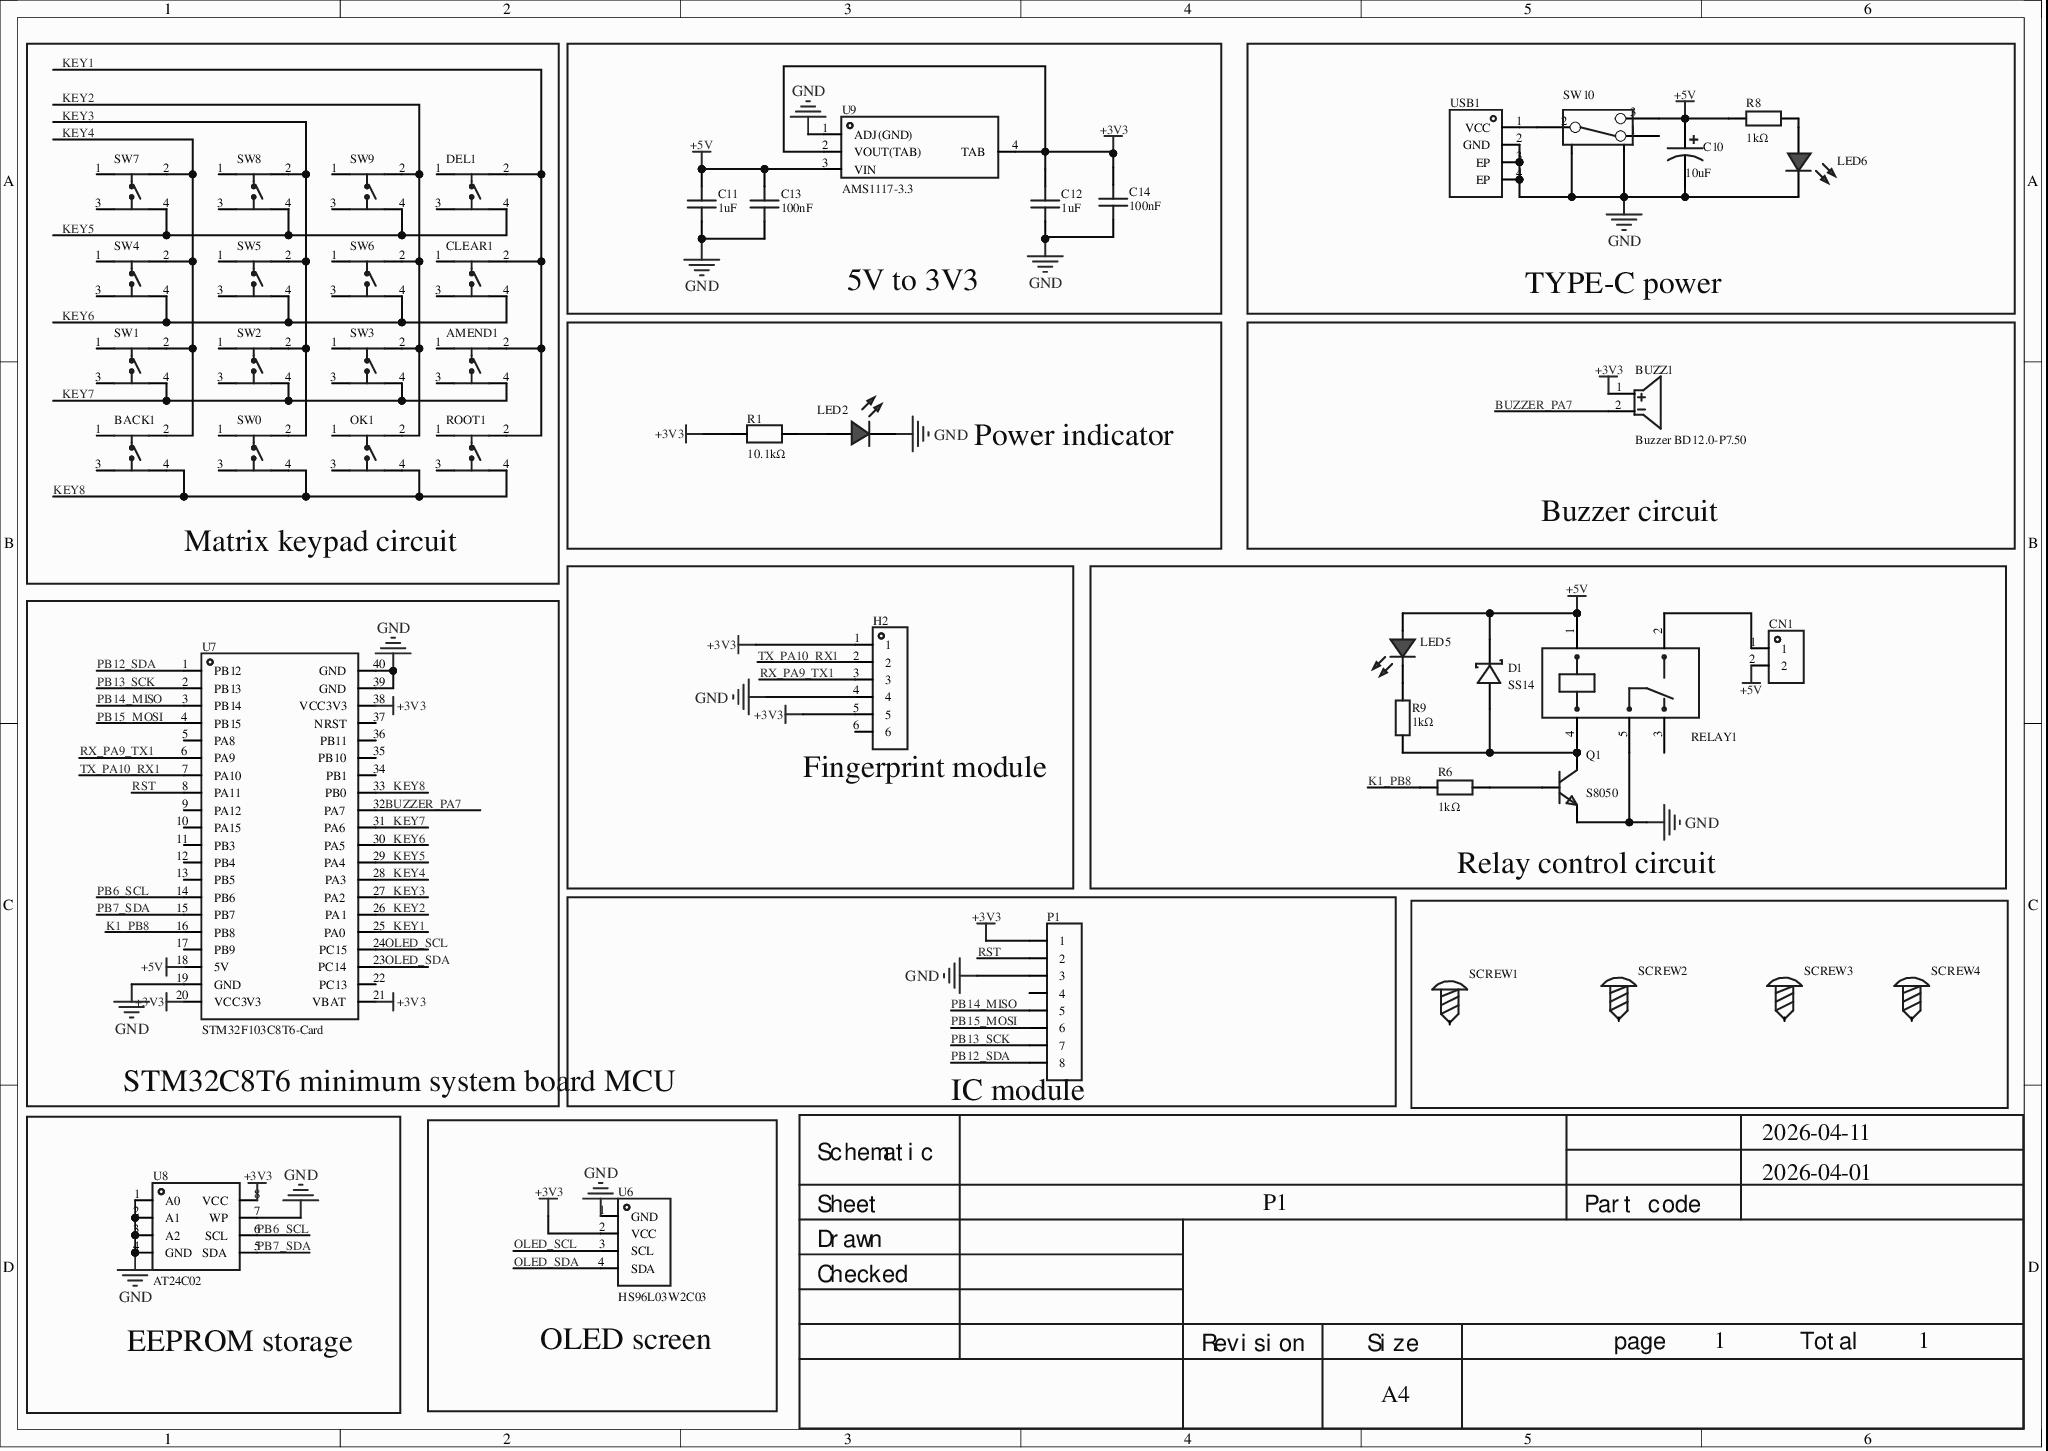
[diagram p0: MISC61668-2.schdoc]
# Altium project MISC61668-3.PrjPcb
1 sheet, 45 parts. Net scope: global (net labels, ports and power ports of the same name join across sheets).
Board file: MISC61668.pcbdoc

## Sheet MISC61668-2.schdoc
size 297 x 210 mm; Version: V1.0; @Project Name: MISC61668; @Page Count: 1; @Update Date: 2026-04-11; @Create Date: 2026-04-11; @Schematic Name: MISC61668; @Page No: 1

### Parts
AMEND1  KH-6X6X5H-STM  [SW-SMD_4P-L6.0-W6.0-P4.50-LS9.0-2]  (value not drawn)
BACK1  KH-6X6X5H-STM  [SW-SMD_4P-L6.0-W6.0-P4.50-LS9.0-2]  (value not drawn)
BUZZ1  Buzzer BD12.0-P7.50  [BUZ-TH_BD12.0-P7.50-D0.6-FD]
C10  10uF  [CAP-TH_BD5.0-P2.00-D0.8-FD]
C11  1uF  [C0603]
C12  1uF  [C0603]
C13  100nF  [C0603]
C14  100nF  [C0603]
CLEAR1  KH-6X6X5H-STM  [SW-SMD_4P-L6.0-W6.0-P4.50-LS9.0-2]  (value not drawn)
CN1  ZX-XH2.54-2PZZ  [CONN-TH_2P-P2.50_HX25003-2A]  (value not drawn)
D1  SS14  [SMA_L4.2-W2.6-LS5.3-RD]
DEL1  KH-6X6X5H-STM  [SW-SMD_4P-L6.0-W6.0-P4.50-LS9.0-2]  (value not drawn)
H2  PM254V-11-06-H85  [hdr-th_6p-p2.54-v-f]  (value not drawn)
LED2  (no value)  [LED-TH_5mm]
LED5  XL-302SURD  [LED-TH_BD3.8-P2.54-RD]  (value not drawn)
LED6  (no value)  [LED-TH_5mm]
OK1  KH-6X6X5H-STM  [SW-SMD_4P-L6.0-W6.0-P4.50-LS9.0-2]  (value not drawn)
P1  2.54-1*8P female, RoHS  [HDR-TH_8P-P2.54-V-F-1]  (value not drawn)
Q1  S8050  [SOT-23-3_L2.9-W1.6-P1.90-LS2.8-BR]
R1  10.1kΩ  [R0805]
R6  1kΩ  [R0603]
R8  1kΩ  [RES-TH_BD2.5-L6.5-P10.50-D0.6]
R9  1kΩ  [RES-TH_BD2.5-L6.5-P10.50-D0.6]
RELAY1  SRD-12VDC-SL-C  [RELAY-TH_SRD-XXVDC-XL-C]  (value not drawn)
ROOT1  KH-6X6X5H-STM  [SW-SMD_4P-L6.0-W6.0-P4.50-LS9.0-2]  (value not drawn)
SCREW1  (no value)  [M3螺丝]
SCREW2  (no value)  [M3螺丝]
SCREW3  (no value)  [M3螺丝]
SCREW4  (no value)  [M3螺丝]
SW0  KH-6X6X5H-STM  [SW-SMD_4P-L6.0-W6.0-P4.50-LS9.0-2]  (value not drawn)
SW1  KH-6X6X5H-STM  [SW-SMD_4P-L6.0-W6.0-P4.50-LS9.0-2]  (value not drawn)
SW2  KH-6X6X5H-STM  [SW-SMD_4P-L6.0-W6.0-P4.50-LS9.0-2]  (value not drawn)
SW3  KH-6X6X5H-STM  [SW-SMD_4P-L6.0-W6.0-P4.50-LS9.0-2]  (value not drawn)
SW4  KH-6X6X5H-STM  [SW-SMD_4P-L6.0-W6.0-P4.50-LS9.0-2]  (value not drawn)
SW5  KH-6X6X5H-STM  [SW-SMD_4P-L6.0-W6.0-P4.50-LS9.0-2]  (value not drawn)
SW6  KH-6X6X5H-STM  [SW-SMD_4P-L6.0-W6.0-P4.50-LS9.0-2]  (value not drawn)
SW7  KH-6X6X5H-STM  [SW-SMD_4P-L6.0-W6.0-P4.50-LS9.0-2]  (value not drawn)
SW8  KH-6X6X5H-STM  [SW-SMD_4P-L6.0-W6.0-P4.50-LS9.0-2]  (value not drawn)
SW9  KH-6X6X5H-STM  [SW-SMD_4P-L6.0-W6.0-P4.50-LS9.0-2]  (value not drawn)
SW10  SK-12E12-G5  [SW-TH_SK-12E12-G5]  (value not drawn)
U6  HS96L03W2C03  [OLED-TH_L27.8-W27.2-P2.54_C9900033791]
U7  STM32F103C8T6-Card  [CONN-TH_L53.3-W22.9_STM32F103C8T6-CARD]
U8  AT24C02  [SOP-8_L5.0-W4.0-P1.27-LS6.0-BL]
U9  AMS1117-3.3  [SOT-223-4_L6.5-W3.5-P2.30-LS7.0-BR]
USB1  KH-TYPE-C-2P  [USB-SMD_KH-TYPE-C-2P]  (value not drawn)

### Blocks framed on the sheet
Matrix keypad circuit: AMEND1 BACK1 CLEAR1 DEL1 OK1 ROOT1 SW0-SW9
5V to 3V3: C11-C14 U9
TYPE-C power: C10 LED6 R8 SW10 USB1
Power indicator: LED2 R1
Fingerprint module: H2
STM32C8T6 minimum system board MCU: U7
IC module: P1
Relay control circuit: SCREW1-SCREW4
OLED screen: U6

### Nets
+3V3: BUZZ1.1 C12.2 C14.2 H2.1 H2.5 P1.1 R1.1 U6.2(VCC) U7.20(VCC3V3) U7.21(VBAT) U7.38(VCC3V3) U8.8(VCC) U9.2(VOUT(TAB)) U9.4(TAB)
+5V: C10.1 C11.2 C13.2 CN1.2 D1.1(K) LED5.2(A) R8.1 RELAY1.1 SW10.3 U7.18(5V) U9.3(VIN)
GND: C10.2 C11.1 C12.1 C13.1 C14.1 H2.4 LED2.2(A) LED6.2(A) P1.3 Q1.2 RELAY1.5 SW10.4 SW10.5 U6.1(GND) U7.19(GND) U7.39(GND) U7.40(GND) U8.1(A0) U8.2(A1) U8.3(A2) U8.4(GND) U8.7(WP) U9.1(ADJ(GND)) USB1.2(GND) USB1.3(EP) USB1.4(EP)
BUZZER_PA7: BUZZ1.2 U7.32(PA7)
K1_PB8: R6.2 U7.16(PB8)
KEY1: AMEND1.2 CLEAR1.2 DEL1.2 ROOT1.2 U7.25(PA0)
KEY2: OK1.2 SW3.2 SW6.2 SW9.2 U7.26(PA1)
KEY3: SW0.2 SW2.2 SW5.2 SW8.2 U7.27(PA2)
KEY4: BACK1.2 SW1.2 SW4.2 SW7.2 U7.28(PA3)
KEY5: DEL1.4 SW7.4 SW8.4 SW9.4 U7.29(PA4)
KEY6: CLEAR1.4 SW4.4 SW5.4 SW6.4 U7.30(PA5)
KEY7: AMEND1.4 SW1.4 SW2.4 SW3.4 U7.31(PA6)
KEY8: BACK1.4 OK1.4 ROOT1.4 SW0.4 U7.33(PB0)
OLED_SCL: U6.3(SCL) U7.24(PC15)
OLED_SDA: U6.4(SDA) U7.23(PC14)
PB6_SCL: U7.14(PB6) U8.6(SCL)
PB7_SDA: U7.15(PB7) U8.5(SDA)
PB12_SDA: P1.8 U7.1(PB12)
PB13_SCK: P1.7 U7.2(PB13)
PB14_MISO: P1.5 U7.3(PB14)
PB15_MOSI: P1.6 U7.4(PB15)
RST: P1.2 U7.8(PA11)
RX_PA9_TX1: H2.3 U7.6(PA9)
TX_PA10_RX1: H2.2 U7.7(PA10)
NetCN1_1: CN1.1 RELAY1.2
NetD1_2: D1.2(A) Q1.3 R9.1 RELAY1.4
NetLED2_1: LED2.1(C) R1.2
NetLED5_1: LED5.1(K) R9.2
NetLED6_1: LED6.1(C) R8.2
NetQ1_1: Q1.1 R6.1
NetSW10_2: SW10.2 USB1.1(VCC)

Not connected (* = marked no-connect by the designer): AMEND1 1* 3*; BACK1 1* 3*; CLEAR1 1* 3*; DEL1 1* 3*; H2 6*; OK1 1* 3*; P1 4*; RELAY1 3*; ROOT1 1* 3*; SCREW1 1*; SCREW2 1*; SCREW3 1*; SCREW4 1*; SW0 1* 3*; SW1 1* 3*; SW2 1* 3*; SW3 1* 3*; SW4 1* 3*; SW5 1* 3*; SW6 1* 3*; SW7 1* 3*; SW8 1* 3*; SW9 1* 3*; SW10 1*; U7 5(PA8)* 9(PA12)* 10(PA15)* 11(PB3)* 12(PB4)* 13(PB5)* 17(PB9)* 22(PC13)* 34(PB1)* 35(PB10)* 36(PB11)* 37(NRST)*

### Notes on the sheet
- Buzzer circuit
- EEPROM storage
- 2026-04-11
- Schematic
- Sheet
- P1
- Part code
- 2026-04-01
- Checked
- Drawn
- Revision
- Size
- A4
- page
- 1
- Total

### Library data of the parts
AMEND1 BACK1 CLEAR1 DEL1 OK1 ROOT1 SW0-SW9 = KH-6X6X5H-STM: 电路结构:单刀单掷;按钮形状:圆形按钮;安装方式:立贴;开关长度:6mm;开关宽度:6mm;开关高度:5mm;带支架:不带;触点电流:50mA;额定电压(DC):12V;机械寿命:8万次;; Manufacturer: kinghelm(金航标); AddInBom: yes; ModelId: fbf4ceca6c4742d48614ab6a891ef981; ModelName: SW-SMD_4P-L6.0-W6.0-P4.50-LS11.0; ModelTransform: 330.708,251.968,0,0,0,0,0,-0.005,0; Circuit: SPST; Actuator Style: Round button; Switch Length: 6mm; Switch Height: 5mm; Strike Gundam: Without; Contact Current: 50mA; Voltage Rating (DC): 12V; Actuator/Cap Color: Black; Pin Style: Gull-wing; Mechanical Life: 8 ten-thousand cycles; Symbol: KH-6X6X5H-STM; Device: KH-6X6X5H-STM; LCSC Part Name: 6*6*5mm 立贴 轻触开关; SupplierPart: C2837531; ManufacturerPart: KH-6X6X5H-STM; Supplier Footprint: SMD; JLCPCB Part Class: Extended library; Datasheet: https://atta.szlcsc.com/upload/public/pdf/source/20210608/C2837531_45E87AB996CE723B09405FF2EA209C4C.pdf; Supplier: LCSC; ConvertToPcb: yes; FootprintName: SW-SMD_4P-L6.0-W6.0-P4.50-LS9.0-2; Mounting Style: SMD; Switch Width: 6mm
BUZZ1 = 蜂鸣器BD12.0-P7.50: AddInBom: yes; ModelId: 0e4a13d1d30a43b48b3e728a221f21ea; ModelTransform: 472.44,472.32441,0,0,0,0,0,0,-137.795; Symbol: Buzzer BD12.0-P7.50; Device: Buzzer BD12.0-P7.50; LCSC Part Name: 蜂鸣器BD12.0-P7.50; SupplierPart: C9900003117; ManufacturerPart: 蜂鸣器BD12.0-P7.50; Supplier Footprint: TH-BD12.0-P7.50-D0.6; JLCPCB Part Class: Extended library; Supplier: LCSC; ConvertToPcb: yes; FootprintName: BUZ-TH_BD12.0-P7.50-D0.6-FD; ModelName: BUZ-TH_BD12.0-P7.50-D0.6-FD
C10 = 01EC1809SHC10UF50V: Capacitance: 10uF; tolerance: ±20%; rated voltage: 50V; ripple current: 50mA@120Hz; ESR: -;; Manufacturer: KNSCHA(科尼盛); AddInBom: yes; ModelId: edeeed87cbc746108d01291548c38636; ModelName: CAP-TH_D5.0×H7.0×P2.0; ModelTransform: 197.091,196.7911,0,0,0,0,0,0,-137.795; φD: 5mm; L: 11mm; Lifetime @ Temp: 5000hrs@105℃; Symbol: 01EC1809SHC10UF50V; Device: 01EC1809SHC10UF50V; LCSC Part Name: 10uF ±20% 50V; SupplierPart: C503219; ManufacturerPart: 01EC1809SHC10UF50V; Supplier Footprint: 插件,D5xL11mm; JLCPCB Part Class: Extended library; Datasheet: https://atta.szlcsc.com/upload/public/pdf/source/20200324/C503219_39D1683F20D4DB1C41D8BE9142629697.pdf; Supplier: LCSC; ConvertToPcb: yes; FootprintName: CAP-TH_BD5.0-P2.00-D0.8-FD; Value: 10uF; Tolerance: ±20%; Rated Voltage: 50V; Ripple Current: 50mA@120Hz; Equivalent Series Resistance(ESR): -; Lead Spacing: 2mm
C11 C12 = CL10A105KB8NNNC: Capacitance: 1uF; tolerance: ±10%; rated voltage: 50V; dielectric (temperature coefficient): X5R;; Manufacturer: SAMSUNG(三星); AddInBom: yes; ModelId: ac125912035d415993ca9572d50418b1; ModelName: C0603_L1.6-W0.8-H0.8; ModelTransform: 62.992,31.496,0,0,0,0,0,0,0; Symbol: CL10A105KB8NNNC; Device: CL10A105KB8NNNC; LCSC Part Name: 1uF ±10% 50V; SupplierPart: C15849; ManufacturerPart: CL10A105KB8NNNC; Supplier Footprint: 0603; JLCPCB Part Class: Basic library; Datasheet: https://atta.szlcsc.com/upload/public/pdf/source/20160218/1457707763339.pdf; Supplier: LCSC; ConvertToPcb: yes; FootprintName: C0603; Value: 1uF; Tolerance: ±10%; Voltage Rated: 50V; Temperature Coefficient: X5R
C13 C14 = CC0603KRX7R9BB104: Capacitance: 100nF; tolerance: ±10%; rated voltage: 50V; dielectric (temperature coefficient): X7R;; Manufacturer: YAGEO(国巨); AddInBom: yes; ModelId: ac125912035d415993ca9572d50418b1; ModelName: C0603_L1.6-W0.8-H0.8; ModelTransform: 62.992,31.496,0,0,0,0,0,0,0; Symbol: CC0603KRX7R9BB104; Device: CC0603KRX7R9BB104; Supplier: LCSC; Manufacturer Part: CC0603KRX7R9BB104; Value: 100nF; Supplier Part: C14663; JLCPCB Part Class: Basic library; LCSC Part Name: 100nF ±10% 50V; Supplier Footprint: 0603; Datasheet: https://atta.szlcsc.com/upload/public/pdf/source/20180910/C282072_33301C7F631E79921B82A8DAC6BCC5B3.pdf; ConvertToPcb: yes; FootprintName: C0603; Tolerance: ±10%; Voltage Rated: 50V; Temperature Coefficient: X7R
CN1 = ZX-XH2.54-2PZZ: 插针结构:1x2P;间距:2.54mm;安装方式:直插;参考系列:XH;总PIN数:2P;排数:1;每排PIN数:2;行距:-;额定电流:3A;触头材质:黄铜;触头镀层:锡;工作温度范围:-25℃~+85℃;; Manufacturer: Megastar(兆星); AddInBom: yes; ModelId: 17c7be61cc0b4bc5acccb67e71c47088; ModelTransform: 295.275,232.283,0,180,0,0,0,-21.654,-129.921; Pins Structure: 1x2P; Pitch: 2.54mm; Reference Series: XH; Number of PINs Per Row: 2; Current Rating (Max): 3A; Symbol: ZX-XH2.54-2PZZ; Device: ZX-XH2.54-2PZZ; LCSC Part Name: ZX-XH2.54-2PZZ; SupplierPart: C7429632; ManufacturerPart: ZX-XH2.54-2PZZ; Supplier Footprint: 插件,P=2.54mm; JLCPCB Part Class: Extended library; Datasheet: https://atta.szlcsc.com/upload/public/pdf/source/20230619/19BA6947230AA44A04D3EDD65E618FD0.pdf; Supplier: LCSC; ConvertToPcb: yes; FootprintName: CONN-TH_2P-P2.50_HX25003-2A; ModelName: CONN-TH_2P-P2.50_HX25003-2A; Mounting Style: Through-hole; Number of Pins: 2P; Number of Rows: 1; Row Spacing: -; Contact Material: Brass; Contact Plating: Tin; Operating Temperature Range: -25℃~+85℃
D1 = SS14_C2480: Diode configuration: independent; forward voltage (Vf): 550mV@1A; DC reverse voltage (Vr): 40V; rectifier current: 1A;; Manufacturer: MDD(辰达半导体); AddInBom: yes; ModelId: c9e8185d46a94015b9fa58a531b156cf; ModelTransform: 204.83943,103.346,0,0,0,0,-0.001,0.001,0; Reverse Leakage Current (Ir): 300uA@40V; Symbol: SS14; Device: SS14_C2480; LCSC Part Name: 电压:40V 电流:1A; SupplierPart: C2480; ManufacturerPart: SS14; Supplier Footprint: SMA(DO-214AC); JLCPCB Part Class: Basic library; Datasheet: https://atta.szlcsc.com/upload/public/pdf/source/20240710/EF24798823EE33D63F154ED67BAC5E71.pdf; Supplier: LCSC; ConvertToPcb: yes; FootprintName: SMA_L4.2-W2.6-LS5.3-RD; ModelName: SMA_L4.2-W2.6-LS5.3-RD; Diode Configuration: Independent; Forward Voltage (Vf@If): 550mV@1A; Reverse Voltage (Vr): 40V; Rectified Current: 1A
H2 = PM254V-11-06-H85: 插孔结构:1x6P;间距:2.54mm;行距:-;圆孔/方孔:方孔;安装类型:直插;排数:单排;总孔位数:6P;额定电流:3A;额定电压:250V;插孔方向:顶部;塑高:-;工作温度范围:-40℃~+105℃;; Manufacturer: XFCN(兴飞); Check: false; AddInBom: yes; ModelId: 0f5bcf94dcda47d085f24cdca1696fe9; ModelTransform: 619.684,94.488,0,0,0,0,0,0,-125.984; Holes Structure: 1x6P; Pitch: 2.54mm; Circular Hole / Square Hole: Square hole; Number of Holes: 6P; Current Rating (Max): 3A; Voltage Rating (Max): 250V; Holes Direction: Top; Symbol: PM254V-11-06-H85; Device: PM254V-11-06-H85; Supplier: LCSC; Supplier Part: C2832269; Manufacturer Part: PM254V-11-06-H85; JLCPCB Part Class: Extended library; LCSC Part Name: 间距:2.54mm 1x6P 直插; Supplier Footprint: 插件,P=2.54mm; Datasheet: https://atta.szlcsc.com/upload/public/pdf/source/20210514/C2832269_B3EC97736B37C2783BDCE3050AA57447.pdf; ConvertToPcb: yes; FootprintName: hdr-th_6p-p2.54-v-f; ModelName: HDR-TH_6P-P2.54-V-F; Row Spacing: -; Mounting Type: Through-hole; Number of Rows: Single row; Insulation Height: -; Operating Temperature Range: -40℃~+105℃
LED2 LED6 = LED_TH-R_5mm: ConvertToPcb: yes; ModelId: fe9cea1bdf7642cd8d9a5077ed0e2b58; ModelName: LED-TH_BD5.9-P2.54-RD_RED; ModelTransform: 222.16,238.98,581.81,180,0,0,-6,0,-220; Symbol: LED_TH-R; Device: LED_TH-R_5mm; AddInBom: yes; FootprintName: LED-TH_5mm; Supplier Footprint: 插件
LED5 = XL-302SURD: 灯头类型:3mm圆形灯头;发光颜色:红色;功率:80mW;正向电流:30mA;主波长:615nm~620nm;透镜颜色:红色透镜;色温:-;发光角度:50°;载带方式:-;工作温度:-25℃~+85℃;; Manufacturer: XINGLIGHT(成兴光); AddInBom: yes; Lamp Holder Type: 3mm round lamp holder; Emitted Color: Red; Power Dissipation: 80mW; Forward Current: 30mA; Peak Wavelength: 625nm; Lens Color: Red lens; Viewing Angle: 50°; ModelId: 6a9b7f7cc45d49ea908a5f911cd0be96; ModelTransform: 134.372,149.6,0,180,0,0,6.89,0,-196.85; Symbol: XL-302SURD; Device: XL-302SURD; LCSC Part Name: XL-302SURD; SupplierPart: C2895470; ManufacturerPart: XL-302SURD; Supplier Footprint: 插件,D=3mm; JLCPCB Part Class: Extended library; Datasheet: https://atta.szlcsc.com/upload/public/pdf/source/20240112/E1E2B82945FD635E4907401DDE6D4922.pdf; Supplier: LCSC; ConvertToPcb: yes; Dominant Wavelength: 615nm~620nm; Color Temperature: -; Mounting Sytle: -; Operating Temperature: -25℃~+85℃; FootprintName: LED-TH_BD3.8-P2.54-RD; ModelName: LED-TH_BD3.8-P2.54-RD
P1 = 2.54-1*8P母环保: Socket structure: 1x8P; pitch: 2.54mm; row spacing: -; mounting type: through-hole; rows: single row; total positions: 8P; plastic height: -; contact material: -; contact plating: -;; Manufacturer: BOOMELE(博穆精密); Symbol: Header-Female-2.54_1x8; AddInBom: yes; ModelId: 0f7e4d9227ef4fa08d5469c22cc70cdb; ModelName: HDR-F-2.54_1x8; ModelTransform: 799.99844,100,0,0,0,0,0,0,-118.11; Device: 2.54-1*8P female, RoHS; LCSC Part Name: 间距:2.54mm 1x8P 直插; SupplierPart: C27438; ManufacturerPart: 2.54-1*8P母环保; Supplier Footprint: 插件,P=2.54mm; JLCPCB Part Class: Extended library; Datasheet: https://atta.szlcsc.com/upload/public/pdf/source/20231221/1CA800C6799ED97958773716FAA1BFFE.pdf; Supplier: LCSC; ConvertToPcb: yes; FootprintName: HDR-TH_8P-P2.54-V-F-1; Holes Structure: 1x8P; Pitch: 2.54mm; Row Spacing: -; Mounting Type: Through-hole; Number of Rows: Single row; Number of Holes: 8P; Insulation Height: -; Contact Material: -; Contact Plating: -
Q1 = S8050_C181158: Transistor type: NPN; collector current (Ic): 500mA; collector-emitter breakdown voltage (Vceo): 25V; power (Pd): 300mW;; Manufacturer: Hottech(合科泰); AddInBom: yes; ModelId: 89cb27a44ab2466697082bb9fd73a7d0; ModelName: SOT-23-3L_L2.9-W1.6-H1.1-LS2.8-P0.95; ModelTransform: 114.173,110.236,0,90,0,0,0,0,0; Transition Frequency (fT): 150MHz; Collector Cut-Off Current (Icbo): 100nA; Collector-Emitter Saturation Voltage (VCE(sat)@Ic,Ib): 600mV@500mA,50mA; Symbol: S8050_C181158; Device: S8050_C181158; LCSC Part Name: NPN 电流:500mA 耐压:25V; SupplierPart: C181158; ManufacturerPart: S8050; Supplier Footprint: SOT-23; JLCPCB Part Class: Extended library; Datasheet: https://atta.szlcsc.com/upload/public/pdf/source/20220506/D987F39D56F2975D34EC7947E75C4ABC.pdf; Supplier: LCSC; ConvertToPcb: yes; FootprintName: SOT-23-3_L2.9-W1.6-P1.90-LS2.8-BR; Transistor Type: NPN; Collector Current (Ic): 500mA; Collector-Emitter Breakdown Voltage (Vceo): 25V; Power Dissipation (Pd): 300mW; Operating Temperature: -
R1 = RT0805BRD0710K1L: Resistor type: thin film; resistance: 10.1kΩ; tolerance: ±0.1%; power: 125mW; temperature coefficient: ±25ppm/℃;; Manufacturer: YAGEO(国巨); AddInBom: yes; ModelId: 37a81e68749a4138bd2dfa6897b24b85; ModelName: R0805_L2.0-W1.3-H0.6; ModelTransform: 78.74,51.181,0,0,0,0,0,-0.0005,0; Symbol: RT0805BRD0710K1L; Device: RT0805BRD0710K1L; LCSC Part Name: 薄膜电阻 10.1kΩ ±0.1% 125mW; SupplierPart: C865133; ManufacturerPart: RT0805BRD0710K1L; Supplier Footprint: 0805; JLCPCB Part Class: Extended library; Datasheet: https://atta.szlcsc.com/upload/public/pdf/source/20200610/C326738_5639A9F1B6EB6E4AE2197577D3456E7F.pdf; Supplier: LCSC; ConvertToPcb: yes; FootprintName: R0805; Type: Thin film resistor; Value: 10.1kΩ; Tolerance: ±0.1%; Power(Watts): 125mW; Temperature Coefficient: ±25ppm/℃; Operating Temperature Range: -55℃~+155℃
R6 = RC0603FR-071KL: Resistor type: thick film; resistance: 1kΩ; tolerance: ±1%; power: 100mW; max working voltage: 75V; temperature coefficient: ±100ppm/℃;; Manufacturer: YAGEO(国巨); AddInBom: yes; ModelId: fc143cca1e79419f9cd78b61e9279f08; ModelTransform: 31.8897,63.7794,0,90,0,0,0,0,0; Symbol: RC0603FR-071KL; Device: RC0603FR-071KL; LCSC Part Name: 厚膜电阻 1kΩ ±1% 100mW; SupplierPart: C22548; ManufacturerPart: RC0603FR-071KL; Supplier Footprint: 0603; JLCPCB Part Class: Extended library; Datasheet: https://atta.szlcsc.com/upload/public/pdf/source/20180316/70C0E2BDAE7FCC62C531A5A58D202EE1.pdf; Supplier: LCSC; ConvertToPcb: yes; FootprintName: R0603; ModelName: R0603; Type: Thick film resistor; Value: 1kΩ; Tolerance: ±1%; Power(Watts): 100mW; Overload Voltage (Max): 75V; Temperature Coefficient: ±100ppm/℃; Operating Temperature Range: -55℃~+155℃
R8 R9 = MFR0W4F1001A50: Resistor type: metal film; resistance: 1kΩ; tolerance: ±1%; power: 250mW; temperature coefficient: ±50ppm/℃;; Manufacturer: UNI-ROYAL(厚声); AddInBom: yes; ModelId: 8e6c7ee8323443d1ab8f0504b6353c8c; ModelName: RES-TH_D2.3-L6.5-P10.50; ModelTransform: 431.1015,91.3384,0,0,0,0,0.197,0,-137.795; Overload Voltage (Max): 250V; Symbol: MFR0W4F1001A50; Device: MFR0W4F1001A50; Supplier: LCSC; Manufacturer Part: MFR0W4F1001A50; Supplier Part: C57435; Value: 1kΩ; JLCPCB Part Class: Extended library; LCSC Part Name: 1kΩ ±1% 250mW 金属膜电阻; Supplier Footprint: 插件; Datasheet: https://atta.szlcsc.com/upload/public/pdf/source/20191012/C436293_8820AA14BC71FA35E551C06C441482A0.pdf; ConvertToPcb: yes; FootprintName: RES-TH_BD2.5-L6.5-P10.50-D0.6; Type: Metal film resistor; Tolerance: ±1%; Power(Watts): 250mW; Temperature Coefficient: ±50ppm/℃
RELAY1 = SRD-12VDC-SL-C: Coil voltage: 12V; contact form: changeover 1C (SPDT); contact rating (resistive load): -; max switching voltage: 250V@AC; max switching current: 15A;; Manufacturer: 松乐; AddInBom: yes; ModelId: d0eda9b8bf8746d18ae810ab88dc78e7; ModelName: RELAY-TH_L19.2-W15.6-H15.8; ModelTransform: 755.904,622.4397,0,0,0,0,34.882,0,-118.11; Pin Number: 5; Coil Rated Power: 360mW; Coil Type: Non-polarized, single coil; Coil Resistance: 400Ω; Contact Resistance: 100mΩ; Operate Time: 10ms; Symbol: SRD-12VDC-SL-C; Device: SRD-12VDC-SL-C; LCSC Part Name: SRD-12VDC-SL-C; SupplierPart: C30431; ManufacturerPart: SRD-12VDC-SL-C; Supplier Footprint: 插件,15.6x19.2mm; JLCPCB Part Class: Extended library; Datasheet: https://atta.szlcsc.com/upload/public/pdf/source/20200305/C490149_C96E4098A3B1FFB377D5AD2E40B7C2A8.pdf; Supplier: LCSC; ConvertToPcb: yes; FootprintName: RELAY-TH_SRD-XXVDC-XL-C; Coil Voltage: 12V; Contact Form: Changeover 1C (SPDT); Contact Rating: -; Maximum Switching Voltage: 250V@AC; Maximum Switching Current: 15A; Release Time: 10ms
SCREW1-SCREW4 = M3螺丝: Device: M3 screw; ConvertToPcb: yes; SymbolName: Screw hole; AddInBom: yes; Supplier Footprint: 插件; FootprintName: M3 screw
SW10 = SK-12E12-G5: Circuit structure: SPDT; mounting style: side entry; rated current (DC): -; rated voltage (DC): -; rated current (AC): -; rated voltage (AC): -; mechanical life: 5 thousand cycles;; Manufacturer: 韩国韩荣; AddInBom: yes; ModelId: 63ecb7c3b60e41c79481f203e3e77e6b; ModelTransform: 507.874,401.575,0,90,0,0,105,0,-137.795; Actuator Style: Rectangular post; Pin Style: PC pin; Switch Height: 10.6mm; Symbol: SK-12E12-G5; Device: SK-12E12-G5; LCSC Part Name: 卧插双档 滑动开关; SupplierPart: C136720; ManufacturerPart: SK-12E12-G5; Supplier Footprint: 插件; JLCPCB Part Class: Extended library; Datasheet: https://atta.szlcsc.com/upload/public/pdf/source/20210810/880D64C2F8CCE477762EFCC00B7B7681.pdf; Supplier: LCSC; ConvertToPcb: yes; FootprintName: SW-TH_SK-12E12-G5; ModelName: SW-TH_SK-12E12-G5; Circuit: SPDT; Mounting Style: Side entry; Current Rating (DC): -; Voltage Rating (DC): -; Current Rating (AC): -; Voltage Rating (AC): -; Mechanical Life: 5 thousand cycles; Operating Temperature: -25℃~+70℃
U6 = HS96L03W2C03: Main controller chip: SSD1315; interface type: I2C; size (inch): 0.96; pixel resolution: 128x64;; Manufacturer: HS(汉昇); AddInBom: yes; ModelId: c6b423183c2f4cf5a163f75f8ad52fae; ModelTransform: 1070.864,1094.486,0,0,0,0,0,-468.503,0; Symbol: HS96L03W2C03; Device: HS96L03W2C03; LCSC Part Name: 0.96寸OLED显示屏窄白光IIC; SupplierPart: C5248080; ManufacturerPart: HS96L03W2C03; Supplier Footprint: -; JLCPCB Part Class: Extended library; Datasheet: https://atta.szlcsc.com/upload/public/pdf/source/20230627/763D01F79A90007632F098068C7C8AD9.pdf; Supplier: LCSC; ConvertToPcb: yes; FootprintName: OLED-TH_L27.8-W27.2-P2.54_C9900033791; ModelName: OLED-TH_L27.8-W27.2-P2.54_C9900033791; Main Control Chip: SSD1315; Interface Type: I2C; Size: 0.96; Pixel Resolution: 128x64; Operating Temperature: -40℃~+70℃
U7 = STM32F103C8T6-Card: AddInBom: yes; Symbol: STM32F103C8T6-CARD; Device: STM32F103C8T6-Card; LCSC Part Name: STM32F103C8T6-Card; SupplierPart: C9900077949; ManufacturerPart: STM32F103C8T6-Card; Supplier Footprint: 插件; JLCPCB Part Class: Extended Part; Supplier: LCSC; ConvertToPcb: yes; FootprintName: CONN-TH_L53.3-W22.9_STM32F103C8T6-CARD
U8 = AT24C02_C688857: Manufacturer: IDCHIP(英锐芯); AddInBom: yes; ModelId: a3315c1c78f949e6bb82c6eaca1c53c7; ModelName: SOP-8_L5.0-W4.0-H1.8-LS6.2-P1.27; ModelTransform: 244.094,196.85,0,90,0,0,0,0,0; Symbol: AT24C02; Device: AT24C02_C688857; LCSC Part Name: AT24C02; SupplierPart: C688857; ManufacturerPart: AT24C02; Supplier Footprint: SOP-8; JLCPCB Part Class: Extended library; Datasheet: https://atta.szlcsc.com/upload/public/pdf/source/20200619/C688857_168265888F77B455D6D4136881F4BB15.pdf; Supplier: LCSC; ConvertToPcb: yes; FootprintName: SOP-8_L5.0-W4.0-P1.27-LS6.0-BL
U9 = AMS1117-3.3_C347222: Output type: fixed; max input voltage: 12V; output voltage: 3.3V; max output current: 1A; PSRR: 60dB@(120Hz); output polarity: positive;; Manufacturer: UMW(友台半导体); AddInBom: yes; ModelId: 925194bf9823436183a3e0b978a8d076; ModelName: SOT-223-4P_L6.5-W3.5-H1.6-LS7.0-P2.30; ModelTransform: 279.89794,255.905,0,180,0,0,-0.0005,-0.0005,0; Dropout Voltage: 1.3V@(1A); Number of Outputs: 1; Symbol: AMS1117-3.3_C347222; Device: AMS1117-3.3_C347222; LCSC Part Name: 输出:3.3V 电流:1A 耐压:12V; SupplierPart: C347222; ManufacturerPart: AMS1117-3.3; Supplier Footprint: SOT-223; JLCPCB Part Class: Extended library; Datasheet: https://atta.szlcsc.com/upload/public/pdf/source/20231109/155D79A26D9DB04352555A58D5969DC8.pdf; Supplier: LCSC; ConvertToPcb: yes; FootprintName: SOT-223-4_L6.5-W3.5-P2.30-LS7.0-BR; Output Type: Fixed; Maximum Input Voltage: 12V; Output Voltage: 3.3V; MAX Output Current: 1A; Power Supply Rejection Ratio (PSRR): 60dB@(120Hz); standby current: -; Noise: -; Feature: -; Operating Temperature: -; Output Polarity: Positive
USB1 = KH-TYPE-C-2P: Connector type: Type-C; standard: -; male/female: -; port count: -; contact count: 2P; mounting: -; rated current - power: -; contact material: -; contact plating: -; operating temperature range: -;; Manufacturer: kinghelm(金航标); AddInBom: yes; ModelId: 4464b34a7d0f48c2b8c2350e914c93f5; ModelTransform: 352.362,255.31449,0,0,0,0,0,-49.213,-98.425; Symbol: KH-TYPE-C-2P; Device: KH-TYPE-C-2P; LCSC Part Name: Type-C; SupplierPart: C2919656; ManufacturerPart: KH-TYPE-C-2P; Supplier Footprint: 插件; JLCPCB Part Class: Extended library; Datasheet: https://atta.szlcsc.com/upload/public/pdf/source/20220707/620587A9E0589B27D96D3CEE595CBC98.pdf; Supplier: LCSC; ConvertToPcb: yes; FootprintName: USB-SMD_KH-TYPE-C-2P; ModelName: USB-SMD_KH-TYPE-C-2P; Connector Type: Type-C; Standard: -; Gender: -; Number of Ports: -; Number of Contacts: 2P; Mounting Style: -; Current Rating - Power (Max): -; Contact Material: -; Contact Plating: -; Operating Temperature Range: -